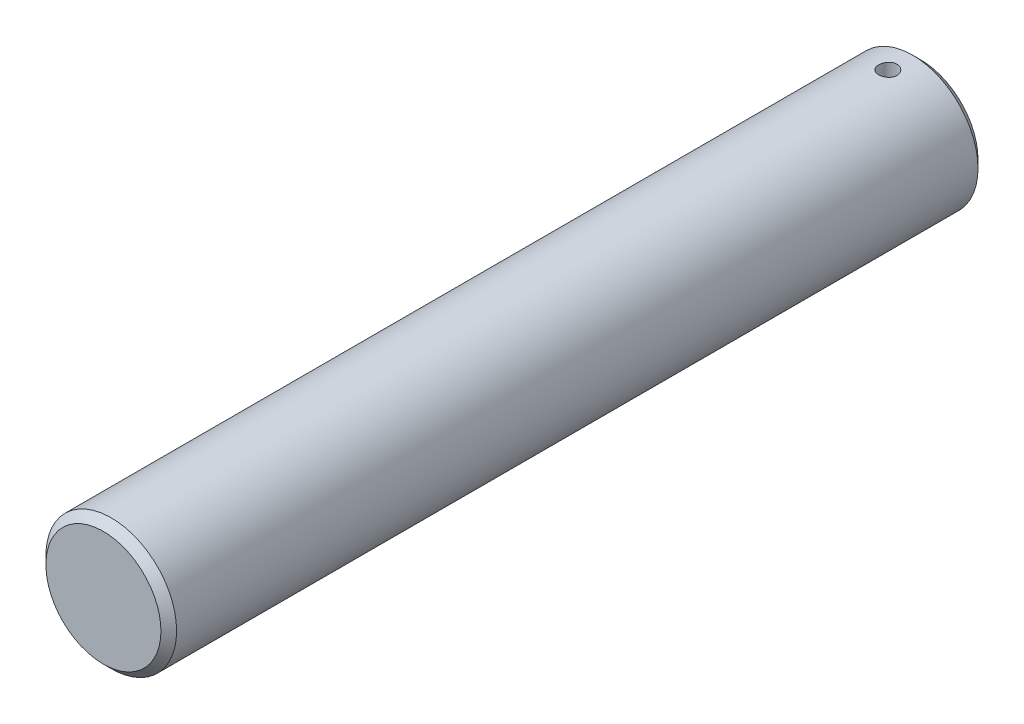
SolidWorks part; units mm, degrees
material "AISI 1020"
ref_plane "Front Plane" through (0, 0, 0) normal (0, 0, 1) x (1, 0, 0)
ref_plane "Top Plane" through (0, 0, 0) normal (0, 1, 0) x (1, 0, 0)
ref_plane "Right Plane" through (0, 0, 0) normal (1, 0, 0) x (0, 0, -1)
sketch "Sketch1" plane through (0, 0, 0) normal (0, 0, 1) x (1, 0, 0)
  circle A0 centre (0, 0) radius 12.7
  dimension "D1" = 25.4
extrude "Boss-Extrude1" add sketch "Sketch1" along normal blind 158.75
chamfer "Chamfer1" distance 1.524 angle 45 2 edges at (12.7, 0, 0) (12.7, 0, 158.75)
sketch "Sketch2" plane through (0, 0, 0) normal (0, 1, 0) x (1, 0, 0)
  line L0 (0, 0) -> (0, -38.5683) construction
  line L1 (-22.6467, -6.35) -> (20.0829, -6.35) construction
  line L2 (11.176, 0) -> (-11.176, 0) construction
  circle A0 centre (0, -6.35) radius 1.785
  dimension "D2" = 3.57
  dimension "D1" = 6.35
extrude "Cut-Extrude1" cut sketch "Sketch2" against normal through all and the other way through all
